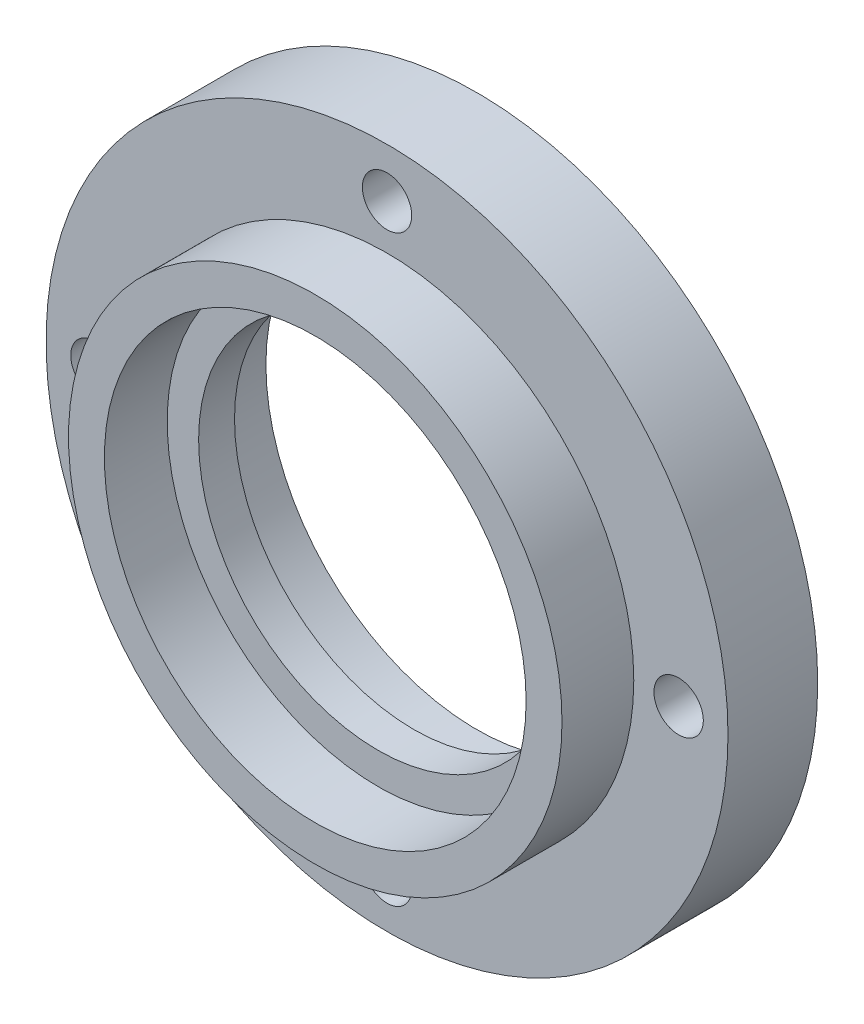
from build123d import *

# Parameters (mm, degrees)
SKETCH1_R                                           = 38
BOSS_EXTRUDE1_DEPTH                                 = 10
SKETCH2_R                                           = 27.5
BOSS_EXTRUDE2_DEPTH                                 = 8
SKETCH3_R                                           = 23.5
CUT_EXTRUDE1_DEPTH                                  = 7
CUT_EXTRUDE2_START                                  = -7
SKETCH4_R                                           = 23.5
CUT_EXTRUDE2_DEPTH                                  = 7
SKETCH6_R                                           = 20
CUT_EXTRUDE3_DEPTH                                  = 57.674509261
CBORE_FOR_M5_HEX_SOCKET_HEAD_CAP_SCREW1_D           = 5.5
CBORE_FOR_M5_HEX_SOCKET_HEAD_CAP_SCREW1_CBORE_D     = 10
CBORE_FOR_M5_HEX_SOCKET_HEAD_CAP_SCREW1_CBORE_DEPTH = 5.4


with BuildPart() as part:
    # Sketch1 → Boss-Extrude1 (new body)
    with BuildSketch(Plane.XY):
        Circle(SKETCH1_R)
    extrude(amount=BOSS_EXTRUDE1_DEPTH)

    # Sketch2 → Boss-Extrude2 (add)
    with BuildSketch(Plane.XY.offset(10)):
        Circle(SKETCH2_R)
    extrude(amount=BOSS_EXTRUDE2_DEPTH)

    # Sketch3 → Cut-Extrude1 (cut)
    with BuildSketch(Plane.XY.offset(18)):
        Circle(SKETCH3_R)
    extrude(amount=-CUT_EXTRUDE1_DEPTH, mode=Mode.SUBTRACT)

    # Sketch4 → Cut-Extrude2 (cut)
    with BuildSketch(Plane(origin=(0, 0, 0), x_dir=(-1, 0, 0), z_dir=(0, 0, -1)).offset(CUT_EXTRUDE2_START)):
        with Locations(Location((0, 0, 0), (0, 0, 180))):
            Circle(SKETCH4_R)
    extrude(amount=CUT_EXTRUDE2_DEPTH, mode=Mode.SUBTRACT)

    # Sketch6 → Cut-Extrude3 (cut, through all)
    with BuildSketch(Plane.XY.offset(18)):
        Circle(SKETCH6_R)
    extrude(amount=-CUT_EXTRUDE3_DEPTH, mode=Mode.SUBTRACT)

    # CBORE for M5 Hex Socket Head Cap Screw1 (through all)
    with Locations(Plane(origin=(0, 0, 0), x_dir=(-1, 0, 0), z_dir=(0, 0, -1))):
        with Locations((0, 32.5), (-32.5, 0), (0, -32.5), (32.5, 0)):
            CounterBoreHole(CBORE_FOR_M5_HEX_SOCKET_HEAD_CAP_SCREW1_D / 2, CBORE_FOR_M5_HEX_SOCKET_HEAD_CAP_SCREW1_CBORE_D / 2, CBORE_FOR_M5_HEX_SOCKET_HEAD_CAP_SCREW1_CBORE_DEPTH)


solid = part.part
